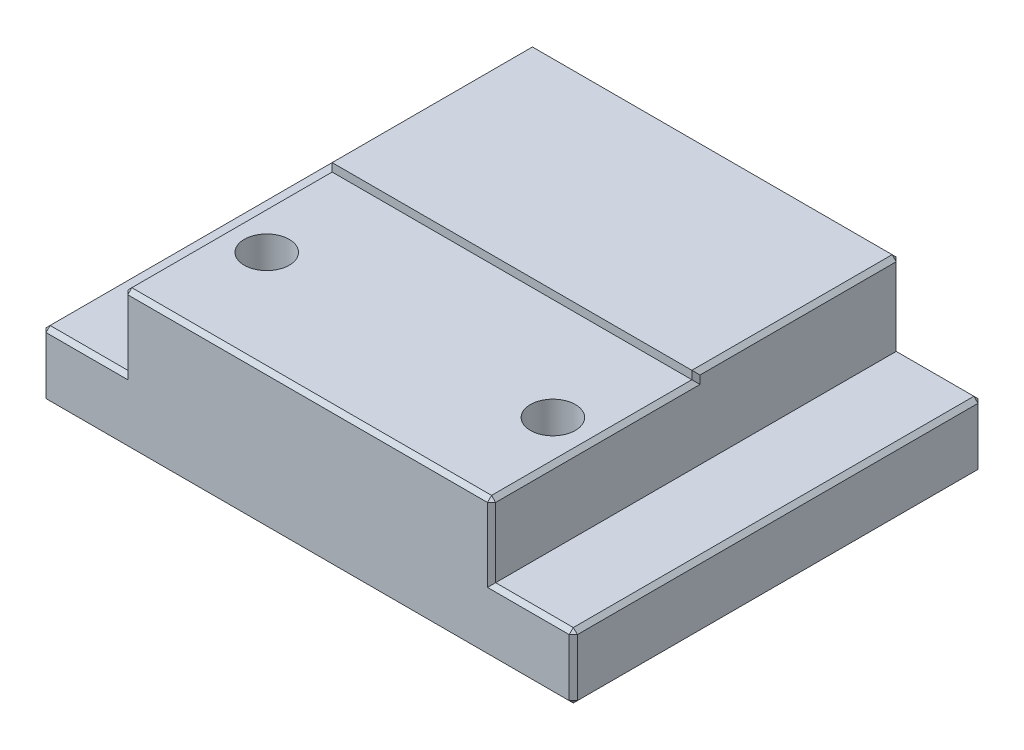
from build123d import *

# Parameters (mm, degrees)
BOSS_EXTRUDE1_DEPTH                          = 50
CBORE_FOR_M5_SLOTTED_CHEESE_HEAD_SCR_2_COUNT = 2
CBORE_FOR_M5_SLOTTED_CHEESE_HEAD_SCR_2_PITCH = 35
SKETCH6_W                                    = 45
SKETCH6_H                                    = 25
CUT_EXTRUDE1_DEPTH                           = 1
CHAMFER1_SIZE                                = 0.5


with BuildPart() as part:
    # Sketch2 → Boss-Extrude1 (new body)
    with BuildSketch(Plane.XY):
        Polygon((55, 8), (65, 8), (65, 0), (0, 0), (0, 8), (10, 8), (10, 18), (55, 18), align=None)
    extrude(amount=BOSS_EXTRUDE1_DEPTH)

    # Sketch4 → CBORE for M5 Slotted cheese head screws1 (revolve, cut)
    with BuildSketch(Plane(origin=(15, 0, 37.5), x_dir=(0, 0, -1), z_dir=(1, 0, 0))):
        Polygon((0, 0), (0, 18), (2.75, 18), (2.75, 6), (5, 6), (5, 0.025), (5.025, 0), align=None)
    cbore_for_m5_slotted_cheese_head_screws1 = revolve(axis=Axis((15, -6.35, 37.5), (0, 1, 0)), mode=Mode.SUBTRACT)

    # CBORE for M5 Slotted cheese head scr 2: CBORE for M5 Slotted cheese head screws1 ×2
    with Locations(*[(i * CBORE_FOR_M5_SLOTTED_CHEESE_HEAD_SCR_2_PITCH, 0, 0) for i in range(1, CBORE_FOR_M5_SLOTTED_CHEESE_HEAD_SCR_2_COUNT)]):
        add(cbore_for_m5_slotted_cheese_head_screws1, mode=Mode.SUBTRACT)

    # Sketch6 → Cut-Extrude1 (cut)
    with BuildSketch(Plane(origin=(0, 18, 0), x_dir=(1, 0, 0), z_dir=(0, 1, 0))):
        with Locations((32.5, -37.5)):
            Rectangle(SKETCH6_W, SKETCH6_H)
    extrude(amount=-CUT_EXTRUDE1_DEPTH, mode=Mode.SUBTRACT)

    # Chamfer1
    chamfer1_edges = [part.edges().sort_by_distance(p)[0] for p in [
        (60, 8, 0),
        (65, 4, 0),
        (32.5, 0, 0),
        (0, 4, 0),
        (65, 4, 50),
        (0, 8, 25),
        (65, 8, 25),
        (65, 0, 25),
        (0, 0, 25),
        (60, 8, 50),
        (55, 12.5, 50),
        (5, 8, 50),
        (10, 12.5, 50),
        (10, 18, 12.5),
        (55, 18, 12.5),
        (0, 4, 50),
        (10, 17, 37.5),
        (10, 17.5, 25),
        (55, 17, 37.5),
        (55, 17.5, 25),
        (32.5, 17, 50),
        (5, 8, 0),
        (32.5, 0, 50),
        (10, 13, 0),
        (32.5, 18, 0),
        (55, 13, 0),
    ]]
    chamfer(chamfer1_edges, length=CHAMFER1_SIZE)


solid = part.part
